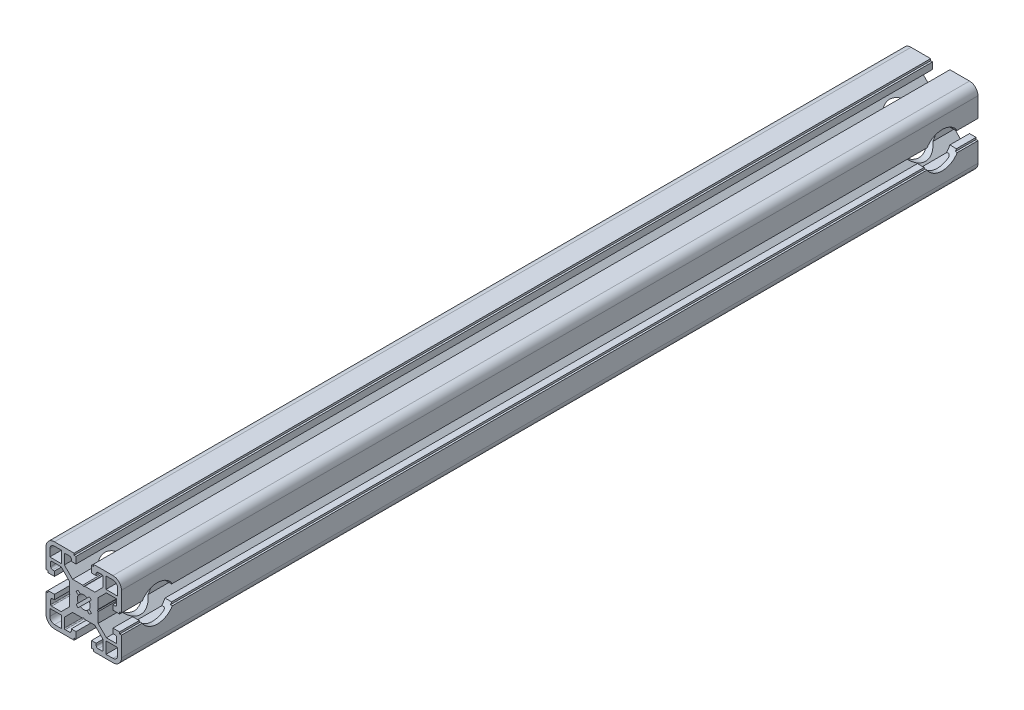
SolidWorks part; units mm, degrees
material "6061 GB/T6892-2006"
ref_plane "前视" through (0, 0, 0) normal (0, 0, 1) x (1, 0, 0)
ref_plane "上视" through (0, 0, 0) normal (0, 1, 0) x (1, 0, 0)
ref_plane "右视" through (0, 0, 0) normal (1, 0, 0) x (0, 0, -1)
sketch "草图1" plane through (0, 0, 0) normal (0, 0, 1) x (1, 0, 0)
  line L0 (-18.9995, -4.1003) -> (-18.9995, -5.1003)
  line L1 (-18.9995, -5.1003) -> (-19.9995, -5.1003)
  line L2 (-19.9995, -5.1003) -> (-19.9995, -15.5003)
  line L3 (-15.4995, -20.0003) -> (-5.0995, -20.0003)
  line L4 (-5.0995, -20.0003) -> (-5.0995, -19.0003)
  line L5 (-5.0995, -19.0003) -> (-4.0995, -19.0003)
  line L6 (-4.0995, -19.0003) -> (-4.0995, -15.5003)
  line L7 (-4.0995, -15.5003) -> (-6.5995, -15.5003)
  line L8 (-6.5995, -15.5003) -> (-6.5995, -16.5003)
  line L9 (-7.5995, -17.5003) -> (-9.7995, -17.5003)
  line L10 (-10.2995, -17.0003) -> (-10.2995, -11.9973)
  line L11 (-10.2995, -11.9973) -> (-5.9025, -7.6003)
  line L12 (-5.9025, -7.6003) -> (-0.5195, -7.6003)
  line L13 (-0.5195, -7.6003) -> (0.0005, -7.3003)
  line L14 (0.0005, -7.3003) -> (0.5195, -7.6003)
  line L15 (0.5195, -7.6003) -> (5.9035, -7.6003)
  line L16 (5.9035, -7.6003) -> (10.3005, -11.9973)
  line L17 (10.3005, -11.9973) -> (10.3005, -17.0003)
  line L18 (9.8005, -17.5003) -> (7.6005, -17.5003)
  line L19 (6.6005, -16.5003) -> (6.6005, -15.5003)
  line L20 (6.6005, -15.5003) -> (4.1005, -15.5003)
  line L21 (4.1005, -15.5003) -> (4.1005, -19.0003)
  line L22 (4.1005, -19.0003) -> (5.1005, -19.0003)
  line L23 (5.1005, -19.0003) -> (5.1005, -20.0003)
  line L24 (5.1005, -20.0003) -> (15.5005, -20.0003)
  line L25 (20.0005, -15.5003) -> (20.0005, -5.1003)
  line L26 (20.0005, -5.1003) -> (19.0005, -5.1003)
  line L27 (19.0005, -5.1003) -> (19.0005, -4.1003)
  line L28 (19.0005, -4.1003) -> (15.5005, -4.1003)
  line L29 (15.5005, -4.1003) -> (15.5005, -6.6003)
  line L30 (15.5005, -6.6003) -> (16.5005, -6.6003)
  line L31 (17.5005, -7.6003) -> (17.5005, -9.8003)
  line L32 (17.0005, -10.3003) -> (11.9975, -10.3003)
  line L33 (11.9975, -10.3003) -> (7.6005, -5.9033)
  line L34 (7.6005, -5.9033) -> (7.6005, -0.5203)
  line L35 (7.6005, -0.5203) -> (7.3005, -0.0003)
  line L36 (7.3005, -0.0003) -> (7.6005, 0.5197)
  line L37 (7.6005, 0.5197) -> (7.6005, 5.9027)
  line L38 (7.6005, 5.9027) -> (11.9975, 10.2997)
  line L39 (11.9975, 10.2997) -> (17.0005, 10.2997)
  line L40 (17.5005, 9.7997) -> (17.5005, 7.5997)
  line L41 (16.5005, 6.5997) -> (15.5005, 6.5997)
  line L42 (15.5005, 6.5997) -> (15.5005, 4.0997)
  line L43 (15.5005, 4.0997) -> (19.0005, 4.0997)
  line L44 (19.0005, 4.0997) -> (19.0005, 5.0997)
  line L45 (19.0005, 5.0997) -> (20.0005, 5.0997)
  line L46 (20.0005, 5.0997) -> (20.0005, 15.4997)
  line L47 (15.5005, 19.9997) -> (5.1005, 19.9997)
  line L48 (5.1005, 19.9997) -> (5.1005, 18.9997)
  line L49 (5.1005, 18.9997) -> (4.1005, 18.9997)
  line L50 (4.1005, 18.9997) -> (4.1005, 15.4997)
  line L51 (4.1005, 15.4997) -> (6.6005, 15.4997)
  line L52 (7.6005, 17.4997) -> (9.8005, 17.4997)
  line L53 (10.3005, 16.9997) -> (10.3005, 11.9967)
  line L54 (10.3005, 11.9967) -> (5.9035, 7.5997)
  line L55 (5.9035, 7.5997) -> (0.5195, 7.5997)
  line L56 (0.5195, 7.5997) -> (0.0005, 7.2997)
  line L57 (0.0005, 7.2997) -> (-0.5195, 7.5997)
  line L58 (-0.5195, 7.5997) -> (-5.9025, 7.5997)
  line L59 (-5.9025, 7.5997) -> (-10.2995, 11.9967)
  line L60 (-10.2995, 11.9967) -> (-10.2995, 16.9997)
  line L61 (-9.7995, 17.4997) -> (-7.5995, 17.4997)
  line L62 (-6.5995, 16.4997) -> (-6.5995, 15.4997)
  line L63 (-6.5995, 15.4997) -> (-4.0995, 15.4997)
  line L64 (-4.0995, 15.4997) -> (-4.0995, 18.9997)
  line L65 (-4.0995, 18.9997) -> (-5.0995, 18.9997)
  line L66 (-5.0995, 18.9997) -> (-5.0995, 19.9997)
  line L67 (-5.0995, 19.9997) -> (-15.4995, 19.9997)
  line L68 (-19.9995, 15.4997) -> (-19.9995, 5.0997)
  line L69 (-19.9995, 5.0997) -> (-18.9995, 5.0997)
  line L70 (-18.9995, 5.0997) -> (-18.9995, 4.0997)
  line L71 (-18.9995, 4.0997) -> (-15.4995, 4.0997)
  line L72 (-15.4995, 4.0997) -> (-15.4995, 6.5997)
  line L73 (-15.4995, 6.5997) -> (-16.4995, 6.5997)
  line L74 (-17.4995, 7.5997) -> (-17.4995, 9.7997)
  line L75 (-16.9995, 10.2997) -> (-11.9965, 10.2997)
  line L76 (-11.9965, 10.2997) -> (-7.5995, 5.9027)
  line L77 (-7.5995, 5.9027) -> (-7.5995, 0.5197)
  line L78 (-7.5995, 0.5197) -> (-7.2995, -0.0003)
  line L79 (-7.2995, -0.0003) -> (-7.5995, -0.5203)
  line L80 (-7.5995, -0.5203) -> (-7.5995, -5.9033)
  line L81 (-7.5995, -5.9033) -> (-11.9965, -10.3003)
  line L82 (-11.9965, -10.3003) -> (-16.9995, -10.3003)
  line L83 (-17.4995, -9.8003) -> (-17.4995, -7.6003)
  line L84 (-16.4995, -6.6003) -> (-15.4995, -6.6003)
  line L85 (-15.4995, -6.6003) -> (-15.4995, -4.1003)
  line L86 (-15.4995, -4.1003) -> (-18.9995, -4.1003)
  line L87 (15.5005, -18.0003) -> (11.8005, -18.0003)
  line L88 (11.8005, -18.0003) -> (11.8005, -11.8003)
  line L89 (11.8005, -11.8003) -> (18.0005, -11.8003)
  line L90 (18.0005, -11.8003) -> (18.0005, -15.5003)
  line L91 (18.0005, 11.7997) -> (11.8005, 11.7997)
  line L92 (11.8005, 11.7997) -> (11.8005, 17.9997)
  line L93 (11.8005, 17.9997) -> (15.5005, 17.9997)
  line L94 (18.0005, 15.4997) -> (18.0005, 11.7997)
  line L95 (-1.8145, -2.8753) -> (-3.0044, -4.0665)
  line L96 (-3.0044, -4.0665) -> (-4.0656, -3.0052)
  line L97 (-4.0656, -3.0052) -> (-2.8745, -1.8153)
  line L98 (-2.8745, 1.8147) -> (-4.0644, 3.0058)
  line L99 (-4.0644, 3.0058) -> (-3.0044, 4.0658)
  line L100 (-3.0044, 4.0658) -> (-1.8145, 2.8747)
  line L101 (1.8145, 2.8747) -> (3.0055, 4.0657)
  line L102 (3.0055, 4.0657) -> (4.0666, 3.0045)
  line L103 (4.0666, 3.0045) -> (2.8755, 1.8147)
  line L104 (2.8755, -1.8153) -> (4.0666, -3.0052)
  line L105 (4.0666, -3.0052) -> (3.0055, -4.0663)
  line L106 (3.0055, -4.0663) -> (1.8145, -2.8753)
  line L107 (-17.9995, -15.5003) -> (-17.9995, -11.8003)
  line L108 (-17.9995, -11.8003) -> (-11.7995, -11.8003)
  line L109 (-11.7995, -11.8003) -> (-11.7995, -18.0003)
  line L110 (-11.7995, -18.0003) -> (-15.4995, -18.0003)
  line L111 (-11.7995, 17.9997) -> (-11.7995, 11.7997)
  line L112 (-11.7995, 11.7997) -> (-17.9995, 11.7997)
  line L113 (-17.9995, 11.7997) -> (-17.9995, 15.4997)
  line L114 (-15.4995, 17.9997) -> (-11.7995, 17.9997)
  arc A0 (-19.9995, -15.5003) -> (-15.4995, -20.0003) centre (-15.4995, -15.5003) ccw
  arc A1 (-6.5995, -16.5003) -> (-7.5995, -17.5003) centre (-7.5995, -16.5003) cw
  arc A2 (-9.7995, -17.5003) -> (-10.2995, -17.0003) centre (-9.7995, -17.0003) cw
  arc A3 (10.3005, -17.0003) -> (9.8005, -17.5003) centre (9.8005, -17.0003) cw
  arc A4 (7.6005, -17.5003) -> (6.6005, -16.5003) centre (7.6005, -16.5003) cw
  arc A5 (15.5005, -20.0003) -> (20.0005, -15.5003) centre (15.5005, -15.5003) ccw
  arc A6 (16.5005, -6.6003) -> (17.5005, -7.6003) centre (16.5005, -7.6003) cw
  arc A7 (17.5005, -9.8003) -> (17.0005, -10.3003) centre (17.0005, -9.8003) cw
  arc A8 (17.0005, 10.2997) -> (17.5005, 9.7997) centre (17.0005, 9.7997) cw
  arc A9 (17.5005, 7.5997) -> (16.5005, 6.5997) centre (16.5005, 7.5997) cw
  arc A10 (20.0005, 15.4997) -> (15.5005, 19.9997) centre (15.5005, 15.4997) ccw
  arc A11 (6.6005, 15.4997) -> (6.6005, 16.4997) centre (7.1003, 15.9997) cw
  arc A12 (6.6005, 16.4997) -> (7.6005, 17.4997) centre (7.6005, 16.4997) cw
  arc A13 (9.8005, 17.4997) -> (10.3005, 16.9997) centre (9.8005, 16.9997) cw
  arc A14 (-10.2995, 16.9997) -> (-9.7995, 17.4997) centre (-9.7995, 16.9997) cw
  arc A15 (-7.5995, 17.4997) -> (-6.5995, 16.4997) centre (-7.5995, 16.4997) cw
  arc A16 (-15.4995, 19.9997) -> (-19.9995, 15.4997) centre (-15.4995, 15.4997) ccw
  arc A17 (-16.4995, 6.5997) -> (-17.4995, 7.5997) centre (-16.4995, 7.5997) cw
  arc A18 (-17.4995, 9.7997) -> (-16.9995, 10.2997) centre (-16.9995, 9.7997) cw
  arc A19 (-16.9995, -10.3003) -> (-17.4995, -9.8003) centre (-16.9995, -9.8003) cw
  arc A20 (-17.4995, -7.6003) -> (-16.4995, -6.6003) centre (-16.4995, -7.6003) cw
  arc A21 (18.0005, -15.5003) -> (15.5005, -18.0003) centre (15.5005, -15.5003) cw
  arc A22 (15.5005, 17.9997) -> (18.0005, 15.4997) centre (15.5005, 15.4997) cw
  arc A23 (-2.8745, -1.8153) -> (-2.8745, 1.8147) centre (0.0005, -0.0003) cw
  arc A24 (-1.8145, 2.8747) -> (1.8145, 2.8747) centre (0, -0.0007) cw
  arc A25 (2.8755, 1.8147) -> (2.8755, -1.8153) centre (0.0005, -0.0003) cw
  arc A26 (1.8145, -2.8753) -> (-1.8145, -2.8753) centre (0, 0) cw
  arc A27 (-15.4995, -18.0003) -> (-17.9995, -15.5003) centre (-15.4995, -15.5003) cw
  arc A28 (-17.9995, 15.4997) -> (-15.4995, 17.9997) centre (-15.4995, 15.4997) cw
extrude "凸台-拉伸1" add sketch "草图1" against normal blind 454
hole_wizard "Ø19.0 (19) 直径孔1" positions "草图2" profile "草图3" hole size "Ø19.0" standard "GB" end condition through all
sketch "草图2" plane through (20.0005, 0, 0) normal (1, 0, 0) x (0, 0, -1)
  line L0 (454, -0.0003) -> (0, -0.0003) construction
  point P0 (19, -0.0003)
  point P4 (435, -0.0003)
  dimension "D1" = 19
  dimension "D2" = 19
sketch "草图3" plane through (20.0005, -0.0003, -19) normal (0, 1, 0) x (0, 0, -1)
  line L0 (0, 0) -> (0, 40)
  line L1 (0, 40) -> (9.5, 40)
  line L2 (9.5, 40) -> (9.5, 0)
  line L5 (9.5, 0) -> (0, 0)
  line L11 (0, -6.35) -> (0, 107.95) construction
  dimension "通孔孔直径" = 19
  dimension "通孔孔深度" = 40
